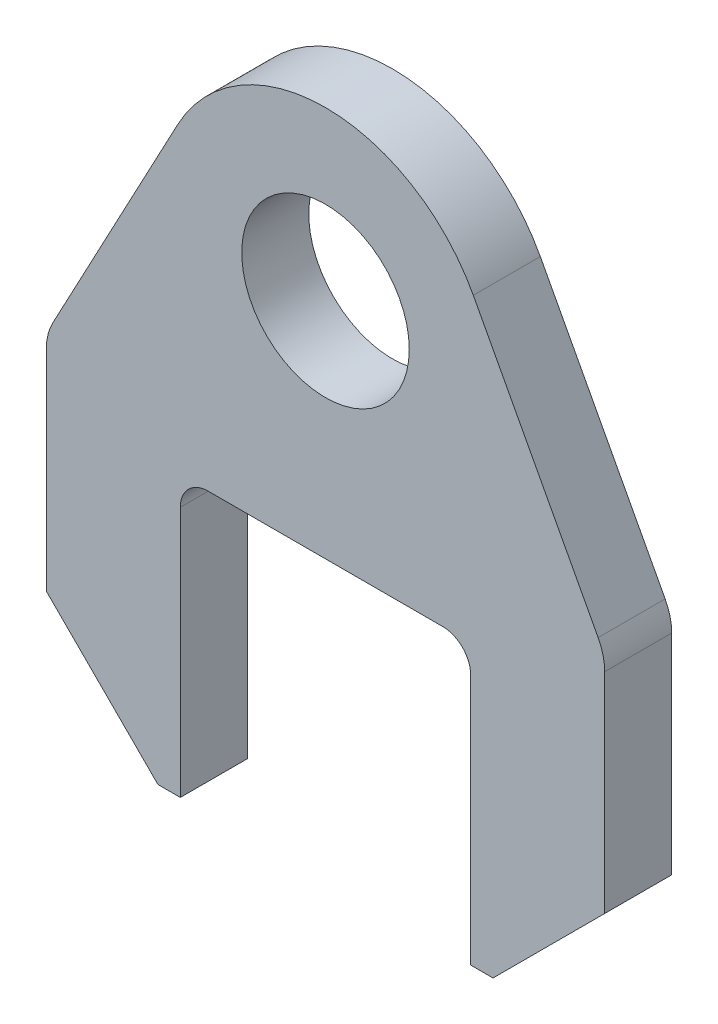
from build123d import *

# Parameters (mm, degrees)
SKETCH1_R           = 15
BOSS_EXTRUDE1_DEPTH = 6


with BuildPart() as part:
    # Sketch1 → Boss-Extrude1 (new, symmetric)
    with BuildSketch(Plane.XY):
        with BuildLine():
            Line((-26, 0), (-30, 0))
            Line((-30, 0), (-50, 20))
            Line((-50, 20), (-50, 57.5))
            ThreePointArc((-50, 57.5), (-49.701425001, 59.92535625), (-48.823529412, 62.205882353))
            Line((-48.823529412, 62.205882353), (-26.470588235, 104.117647059))
            ThreePointArc((-26.470588235, 104.117647059), (0, 120), (26.470588235, 104.117647059))
            Line((26.470588235, 104.117647059), (48.823529412, 62.205882353))
            ThreePointArc((48.823529412, 62.205882353), (49.701425001, 59.92535625), (50, 57.5))
            Line((50, 57.5), (50, 20))
            Line((50, 20), (30, 0))
            Line((30, 0), (26, 0))
            Line((26, 0), (26, 45))
            ThreePointArc((26, 45), (24.535533906, 48.535533906), (21, 50))
            Line((21, 50), (-21, 50))
            ThreePointArc((-21, 50), (-24.535533906, 48.535533906), (-26, 45))
            Line((-26, 45), (-26, 0))
        make_face()
        with Locations((0, 90)):
            Circle(SKETCH1_R, mode=Mode.SUBTRACT)
    extrude(amount=BOSS_EXTRUDE1_DEPTH, both=True)


solid = part.part
